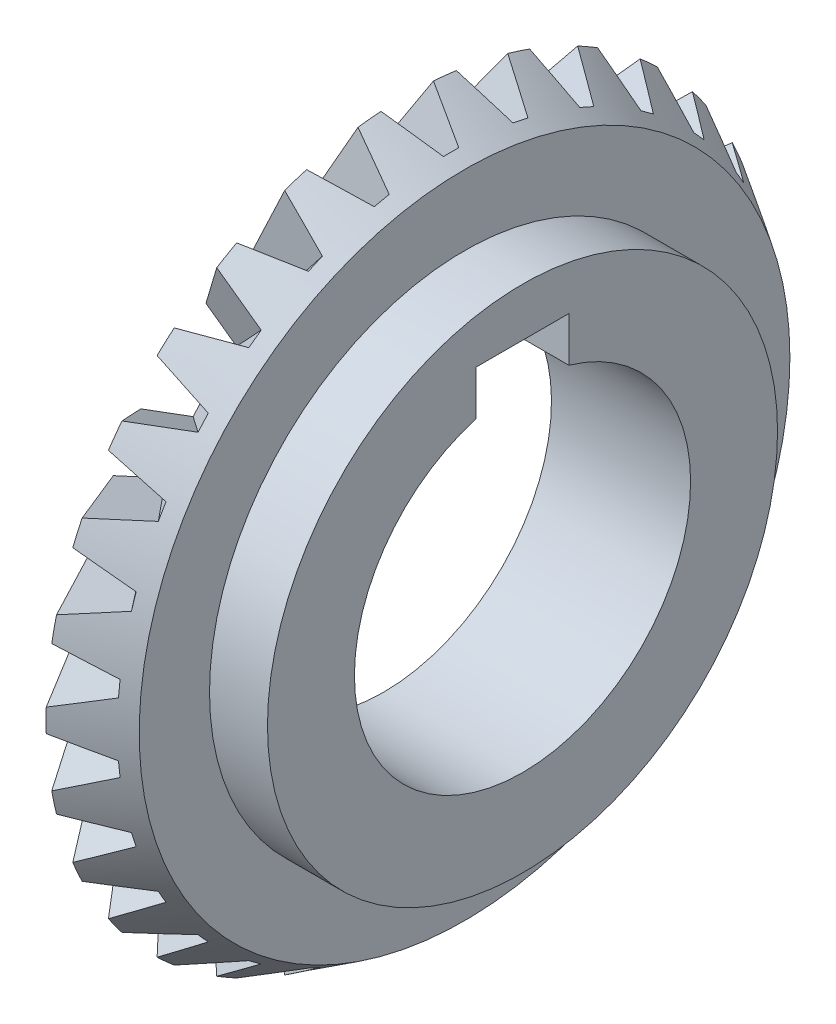
SolidWorks part; units mm, degrees
ref_plane "Front Plane" through (0, 0, 0) normal (0, 0, 1) x (1, 0, 0)
ref_plane "Top Plane" through (0, 0, 0) normal (0, 1, 0) x (1, 0, 0)
ref_plane "Right Plane" through (0, 0, 0) normal (1, 0, 0) x (0, 0, -1)
other "Configuration Table"
sketch "Sketch1" plane through (0, 0, 0) normal (0, 0, 1) x (1, 0, 0)
  line L0 (0, 0) -> (-48.6734, 0) construction
  line L1 (0, 14.5) -> (0, 22)
  line L2 (0, 22) -> (-5, 22)
  line L3 (-5, 22) -> (-5, 28.0664)
  line L4 (-5, 28.0664) -> (-9.9482, 31.15)
  line L5 (-9.9482, 31.15) -> (-16, 21.4387)
  line L6 (-16, 21.4387) -> (-12, 18.946)
  line L7 (-12, 18.946) -> (-12, 14.5)
  line L8 (-12, 14.5) -> (0, 14.5)
  line L9 (-9.9482, 31.15) -> (-29.36, 0) construction
  point P5 (-29.36, 0)
  dimension "D1" = 62.3
  dimension "D2" = 44
  dimension "D4" = 5
  dimension "D5" = 12
  dimension "D6" = 4
  dimension "D7" = 29
  dimension "D8" = 29.36
  dimension "D9" = 58.07
revolve "Revolve1" add sketch "Sketch1" angle 360 about L0
sketch "Sketch2" plane through (0, 0, 0) normal (0, 0, 1) x (1, 0, 0)
  line L0 (-8.2775, 30.1089) -> (-29.36, 0) construction
  line L1 (-5, 28.0664) -> (-9.9482, 31.15) construction
  line L2 (-29.36, 0) -> (0, 0) construction
  line L3 (0, -22) -> (0, 22) construction
  dimension "D1" = 55
  dimension "D2" = 29.36
ref_plane "Plane1" through (-8.2775, 30.1089, 0) normal (0.5289, 0.8487, 0) x (0.8487, -0.5289, 0)
sketch "Sketch3" plane through (-8.2775, 30.1089, 0) normal (0.5289, 0.8487, 0) x (0.8487, -0.5289, 0)
  line L0 (-6.8399, 4.0595) -> (-6.8399, -4.0595)
  line L1 (-6.8399, -4.0595) -> (2.5, -0.6601)
  line L2 (2.5, -0.6601) -> (2.5, 0.6601)
  line L3 (2.5, 0) -> (-27.4663, 0) construction
  line L4 (0, -1.57) -> (0, 1.57) construction
  line L5 (-6.8399, 4.0595) -> (2.5, 0.6601)
  point P9 (0, 0)
  point P11 (-6.8399, 0)
  dimension "D1" = 20
  dimension "D2" = 3.14
  dimension "D3" = 2.5
sketch "Sketch4" plane through (0, 0, 0) normal (0, 0, 1) x (1, 0, 0)
  point P0 (-29.36, 0)
loft "Cut-Loft1" cut profiles "Sketch4", "Sketch3"
pattern_circular "CirPattern1" count 30 over 360 about axis through (0, 0, 0) along (1, 0, 0) of "Cut-Loft1"
sketch "Sketch5" plane through (-12, 0, 0) normal (-1, 0, 0) x (0, 0, 1)
  line L0 (0, 14.5) -> (0, 0) construction
  line L1 (-4, 17.8) -> (4, 17.8)
  line L2 (-4, 17.8) -> (-4, 11.2)
  line L3 (-4, 11.2) -> (4, 11.2)
  line L4 (4, 17.8) -> (4, 11.2)
  line L5 (-4, 17.8) -> (4, 11.2) construction
  line L6 (-4, 11.2) -> (4, 17.8) construction
  circle A0 centre (0, 0) radius 14.5 construction
  point P0 (0, 14.5)
  dimension "D1" = 17.8
  dimension "D2" = 8
extrude "Cut-Extrude1" cut sketch "Sketch5" against normal blind 30
